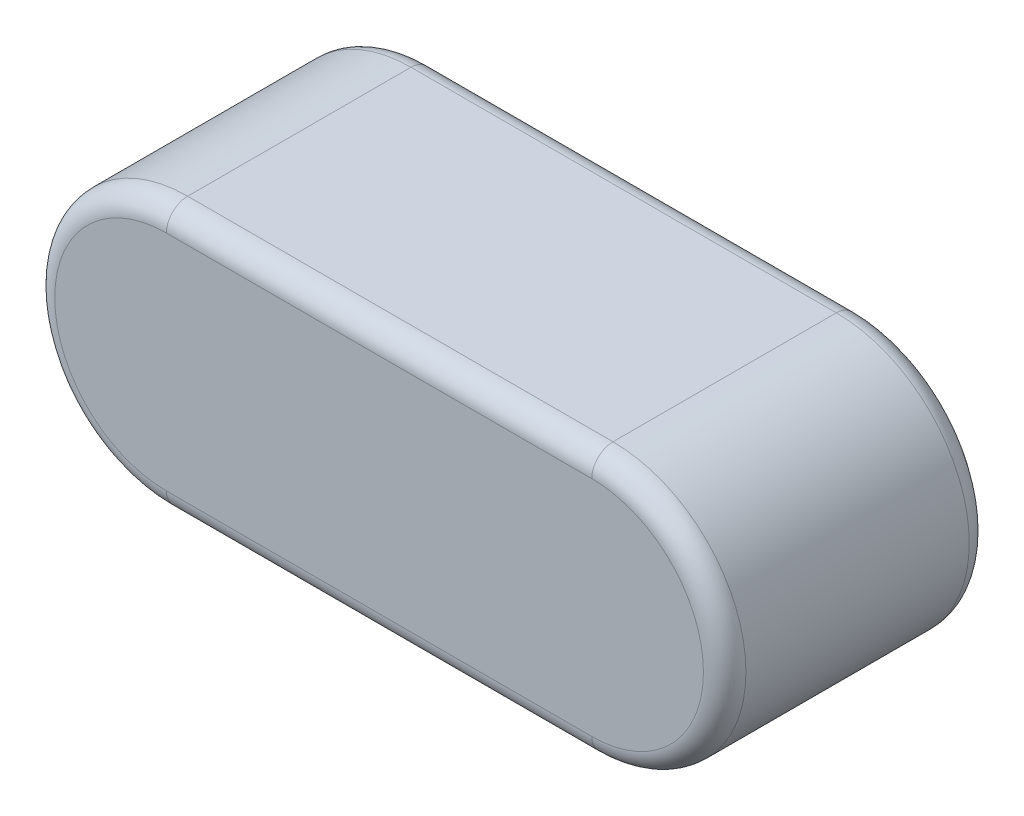
SolidWorks part; units mm, degrees
ref_plane "Plane1" through (0, 0, 0) normal (0, 0, 1) x (1, 0, 0)
ref_plane "Plane2" through (0, 0, 0) normal (0, 1, 0) x (1, 0, 0)
ref_plane "Plane3" through (0, 0, 0) normal (1, 0, 0) x (0, 0, -1)
sketch "Dimension sketch" plane through (0, 0, 0) normal (0, 0, 1) x (1, 0, 0)
  line L0 (-5, 0) -> (5, 0) construction
  point P3 (-5, 0)
  point P4 (-0.4, 0)
  point P5 (0, 0)
  point P8 (-5, 0)
  point P11 (0, 0)
sketch "Sketch1" plane through (0, 0, 0) normal (0, 0, 1) x (1, 0, 0)
  line L0 (-28.0599, 0) -> (30.562, 0) construction
  line L1 (-4, 2.5) -> (4, 2.5)
  line L2 (-4, -2.5) -> (4, -2.5)
  line L3 (0, 2.9108) -> (0, -2.1805) construction
  arc A0 (-4, 2.5) -> (-4, -2.5) centre (-4, 0) ccw
  arc A1 (4, 2.5) -> (4, -2.5) centre (4, 0) cw
extrude "Base-Extrude" add sketch "Sketch1" along normal blind 5
fillet "Fillet1" radius 0.4 8 edges at (6.5, 0, 5) (0, 2.5, 5) (-6.5, 0, 5) (0, 2.5, 0) (6.5, 0, 0) (0, -2.5, 0) (-6.5, 0, 0) (0, -2.5, 5)
equation "\"D1@Sketch1\" = \"b@Dimension sketch\" / 2"
equation "\"D1@Fillet1\" = \"r@Dimension sketch\""
equation "\"D1@Base-Extrude\" = \"h@Dimension sketch\""
